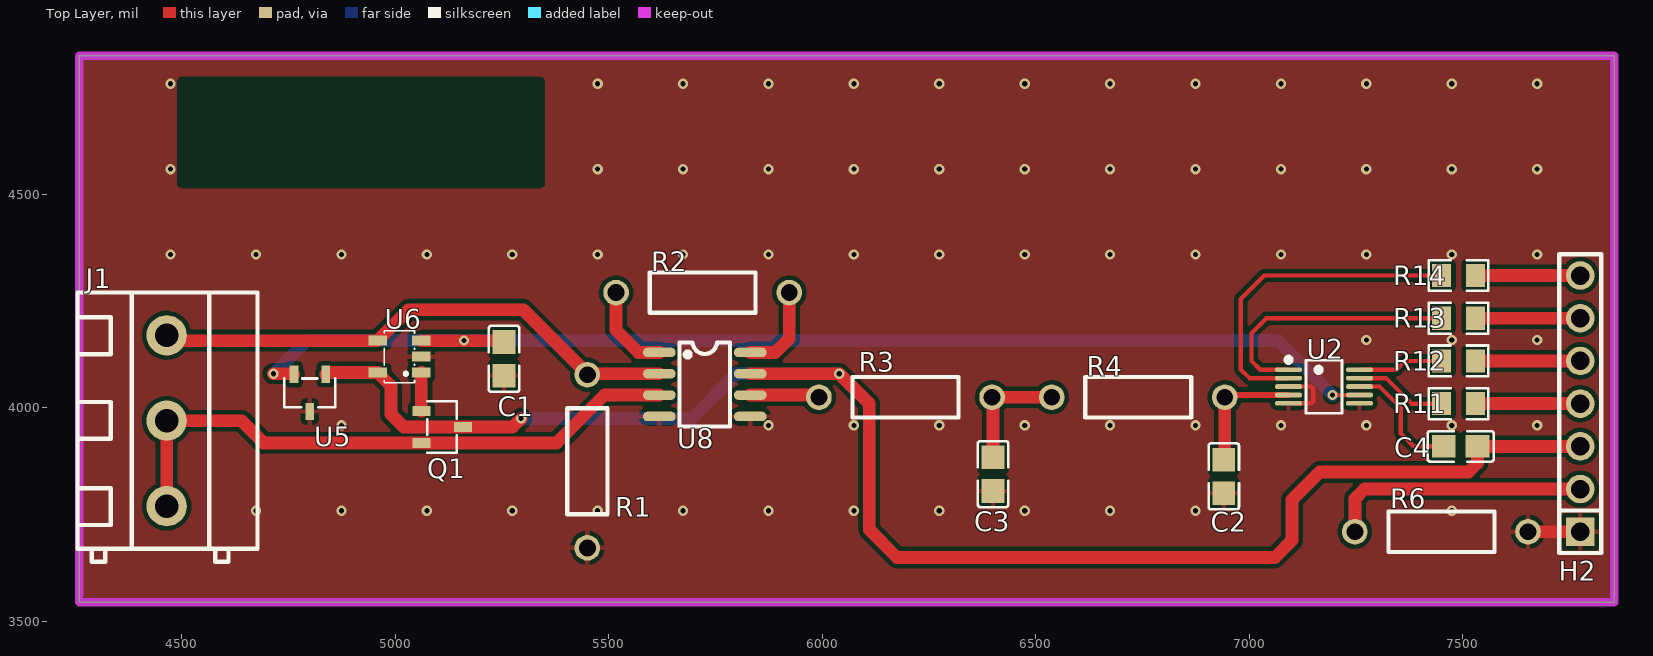
[diagram p0: Top Layer view]
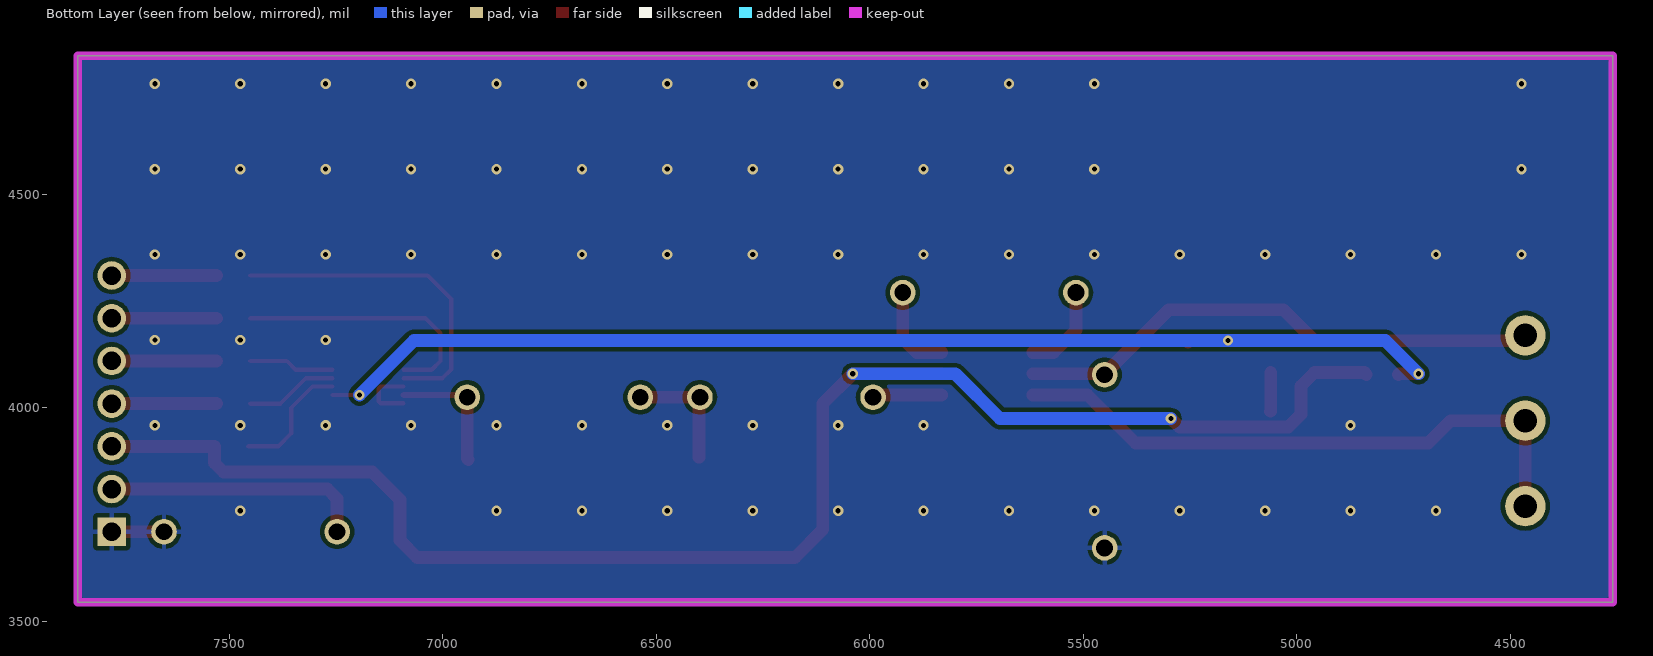
[diagram p1: Bottom Layer view, seen from below]
# Altium PCB MISC51892.pcbdoc
Units mil, origin at the board's own origin, x right, y up, seen from the top; angles counter-clockwise.
Board outline 3595 x 1280 mil, 2 copper layers (Top Layer, Bottom Layer), stack 62.206 mil thick; 20 components, 21 nets, 65 pads, 75 vias.

## Layer stack, top to bottom
Top Solder Mask Layer: solder mask 0.394, Dk 3.3
Top Layer: signal copper 1.379
Dielectric1: surface 59.449, FR4, Dk 4.5
Bottom Layer: signal copper 1.378
Bottom Solder Mask Layer: solder mask 0.394, Dk 3.3

## Board outline
4260,4825 4260,3545 7855,3545 7855,4825

## Design rules (kind name [scope] priority, off if disabled: settings)
BoardOutlineClearance copperThickness2oz_1 [All] p2 off: genericclearance=7.99 ignorepadtopadclearanceinfootprint=FALSE except(0: Arc-SplitContinuation Track-SplitContinuation SMDPad-SplitContinuation THPad-SplitContinuation Via-SplitContinuation Fill-SplitContinuation Region-SplitContinuation Poly-SplitContinuation Text-SplitContinuation Hole-SplitContinuation; 5.98: Arc-CutoutEdge Track-CutoutEdge SMDPad-CutoutEdge THPad-CutoutEdge Via-CutoutEdge Text-CutoutEdge; 6.9: Hole-OutlineEdge Hole-CutoutEdge; 10: Poly-OutlineEdge Poly-CutoutEdge; 11.81: Arc-OutlineEdge Track-OutlineEdge SMDPad-OutlineEdge THPad-OutlineEdge Via-OutlineEdge Fill-OutlineEdge Region-OutlineEdge Text-OutlineEdge Fill-CutoutEdge Region-CutoutEdge)
BoardOutlineClearance Plane_innerPlane_1 [All] p4 off: genericclearance=4.02 ignorepadtopadclearanceinfootprint=FALSE except(0: Arc-SplitContinuation Track-SplitContinuation SMDPad-SplitContinuation THPad-SplitContinuation Via-SplitContinuation Fill-SplitContinuation Region-SplitContinuation Poly-SplitContinuation Text-SplitContinuation Hole-SplitContinuation; 5.98: Arc-CutoutEdge Track-CutoutEdge SMDPad-CutoutEdge THPad-CutoutEdge Via-CutoutEdge Text-CutoutEdge; 6.9: Hole-OutlineEdge Hole-CutoutEdge; 10: Poly-OutlineEdge Poly-CutoutEdge; 11.81: Arc-OutlineEdge Track-OutlineEdge SMDPad-OutlineEdge THPad-OutlineEdge Via-OutlineEdge Fill-OutlineEdge Region-OutlineEdge Text-OutlineEdge Fill-CutoutEdge Region-CutoutEdge)
BoardOutlineClearance Copper_copperRegion_1 [All] p6 off: genericclearance=4.02 ignorepadtopadclearanceinfootprint=FALSE except(0: Arc-SplitContinuation Track-SplitContinuation SMDPad-SplitContinuation THPad-SplitContinuation Via-SplitContinuation Fill-SplitContinuation Region-SplitContinuation Poly-SplitContinuation Text-SplitContinuation Hole-SplitContinuation; 5.98: Arc-CutoutEdge Track-CutoutEdge SMDPad-CutoutEdge THPad-CutoutEdge Via-CutoutEdge Text-CutoutEdge; 6.9: Hole-OutlineEdge Hole-CutoutEdge; 10: Poly-OutlineEdge Poly-CutoutEdge; 11.81: Arc-OutlineEdge Track-OutlineEdge SMDPad-OutlineEdge THPad-OutlineEdge Via-OutlineEdge Fill-OutlineEdge Region-OutlineEdge Text-OutlineEdge Fill-CutoutEdge Region-CutoutEdge)
BoardOutlineClearance copperThickness1oz_1 [All] p8: genericclearance=4.02 ignorepadtopadclearanceinfootprint=FALSE except(0: Arc-SplitContinuation Track-SplitContinuation SMDPad-SplitContinuation THPad-SplitContinuation Via-SplitContinuation Fill-SplitContinuation Region-SplitContinuation Poly-SplitContinuation Text-SplitContinuation Hole-SplitContinuation; 5.98: Arc-CutoutEdge Track-CutoutEdge SMDPad-CutoutEdge THPad-CutoutEdge Via-CutoutEdge Text-CutoutEdge; 6.9: Hole-OutlineEdge Hole-CutoutEdge; 10: Poly-OutlineEdge Poly-CutoutEdge; 11.81: Arc-OutlineEdge Track-OutlineEdge SMDPad-OutlineEdge THPad-OutlineEdge Via-OutlineEdge Fill-OutlineEdge Region-OutlineEdge Text-OutlineEdge Fill-CutoutEdge Region-CutoutEdge)
Clearance copperThickness2oz [All] p1 off: gap=7.99 ignorepadtopadclearanceinfootprint=FALSE except(5.98: SMDPad-Track SMDPad-SMDPad THPad-Track SMDPad-THPad THPad-THPad Track-Via SMDPad-Via THPad-Via Via-Via Fill-SMDPad Region-SMDPad Fill-THPad Region-THPad Fill-Via Region-Via Fill-Fill Fill-Region Region-Region Arc-Track Arc-SMDPad Arc-THPad Arc-Via Fill-Arc Region-Arc Arc-Arc Text-Track SMDPad-Text Text-THPad Text-Via Fill-Text Region-Text Arc-Text Text-Text; 6.9: Hole-Track Hole-SMDPad Hole-THPad Hole-Via Fill-Hole Region-Hole Hole-Arc Hole-Text; 10: Poly-Track Poly-SMDPad Poly-THPad Poly-Via Poly-Fill Poly-Region Poly-Poly Poly-Arc Poly-Text Poly-Hole; 11.81: Fill-Track Region-Track)
Clearance Plane_innerPlane [All] p3 off: gap=4.02 ignorepadtopadclearanceinfootprint=FALSE except(5.98: SMDPad-Track SMDPad-SMDPad THPad-Track SMDPad-THPad THPad-THPad Track-Via SMDPad-Via THPad-Via Via-Via Fill-SMDPad Region-SMDPad Fill-THPad Region-THPad Fill-Via Region-Via Fill-Fill Fill-Region Region-Region Arc-Track Arc-SMDPad Arc-THPad Arc-Via Fill-Arc Region-Arc Arc-Arc Text-Track SMDPad-Text Text-THPad Text-Via Fill-Text Region-Text Arc-Text Text-Text; 6.9: Hole-Track Hole-SMDPad Hole-THPad Hole-Via Fill-Hole Region-Hole Hole-Arc Hole-Text; 10: Poly-Track Poly-SMDPad Poly-THPad Poly-Via Poly-Fill Poly-Region Poly-Poly Poly-Arc Poly-Text Poly-Hole; 11.81: Fill-Track Region-Track)
Clearance Copper_copperRegion [All] p5 off: gap=4.02 ignorepadtopadclearanceinfootprint=FALSE except(5.98: SMDPad-Track SMDPad-SMDPad THPad-Track SMDPad-THPad THPad-THPad Track-Via SMDPad-Via THPad-Via Via-Via Fill-SMDPad Region-SMDPad Fill-THPad Region-THPad Fill-Via Region-Via Fill-Fill Fill-Region Region-Region Arc-Track Arc-SMDPad Arc-THPad Arc-Via Fill-Arc Region-Arc Arc-Arc Text-Track SMDPad-Text Text-THPad Text-Via Fill-Text Region-Text Arc-Text Text-Text; 6.9: Hole-Track Hole-SMDPad Hole-THPad Hole-Via Fill-Hole Region-Hole Hole-Arc Hole-Text; 10: Poly-Track Poly-SMDPad Poly-THPad Poly-Via Poly-Fill Poly-Region Poly-Poly Poly-Arc Poly-Text Poly-Hole; 11.81: Fill-Track Region-Track)
Clearance copperThickness1oz [All] p7: gap=4.02 ignorepadtopadclearanceinfootprint=FALSE except(5.98: SMDPad-Track SMDPad-SMDPad THPad-Track SMDPad-THPad THPad-THPad Track-Via SMDPad-Via THPad-Via Via-Via Fill-SMDPad Region-SMDPad Fill-THPad Region-THPad Fill-Via Region-Via Fill-Fill Fill-Region Region-Region Arc-Track Arc-SMDPad Arc-THPad Arc-Via Fill-Arc Region-Arc Arc-Arc Text-Track SMDPad-Text Text-THPad Text-Via Fill-Text Region-Text Arc-Text Text-Text; 6.9: Hole-Track Hole-SMDPad Hole-THPad Hole-Via Fill-Hole Region-Hole Hole-Arc Hole-Text; 10: Poly-Track Poly-SMDPad Poly-THPad Poly-Via Poly-Fill Poly-Region Poly-Poly Poly-Arc Poly-Text Poly-Hole; 11.81: Fill-Track Region-Track)
DiffPairsRouting differentialPair [All] p1: maxlimit=6 minlimit=6 mostfreqgap=6 toplayer_minwidth=5 toplayer_prefwidth=10 toplayer_maxwidth=100 toplayer_mingap=6 toplayer_prefgap=6 toplayer_maxgap=6 bottomlayer_minwidth=5 bottomlayer_prefwidth=10 bottomlayer_maxwidth=100 bottomlayer_mingap=6 bottomlayer_prefgap=6 bottomlayer_maxgap=6 maxuncoupledlength=10
HoleToHoleClearance otherClearance [All] p1: gap=11.81 allowstackedmicrovias=TRUE
Length netLength [All] p1: minlimit=0 maxlimit=0
PasteMaskExpansion pasteMaskExpansion [All] p1: expansion=0
PlaneConnect innerPlane [All] p1: planeconnectstyle=Relief reliefexpansion=20 reliefentries=4 reliefconductorwidth=10 reliefairgap=10
PolygonConnect copperRegion [All] p1: connectstyle=Relief reliefconductorwidth=10 reliefentries=4 polygonreliefangle="90 Angle" airgapwidth=10 via.connectstyle=Relief via.reliefconductorwidth=10 via.reliefentries=4 via.polygonreliefangle="90 Angle" via.airgapwidth=10
RoutingVias viaSize [All] p1: holewidth=12.01 width=24.02 viastyle="Through Hole" minholewidth=11.81 minwidth=19.68 maxholewidth=248.03 maxwidth=393.7
SolderMaskExpansion solderMaskExpansion [IsVia] p1: expansion=-1000 istentingtop=TRUE
SolderMaskExpansion solderMaskExpansion [All] p2: expansion=2 istentingtop=FALSE
Width copperThickness2oz_2 [All] p1 off: maxlimit=100 minlimit=8 preferedwidth=10
Width copperThickness1oz_2 [All] p2: maxlimit=100 minlimit=5 preferedwidth=10

## Components (designator, comment, footprint, x,y, rotation, side; value= is the part's Value field where it differs from the comment)
C1 "100nF" C0805 5255,4115 r90 top
C2 "100nF" C0805 6940.31,3839.57 r90 top
C3 "100nF" C0805 6400,3845 r90 top
C4 "100nF" C0805 7495,3910 r0 top
H2 "PZ254V-11-07P" HDR-TH_7P-P2.54-V-M 7775,4010 r90 top
J1 "KF128-5.08-3P-AA" CONN-TH_3P-P5.08_KF128-5.08-3P 4465,3970 r270 top
Q1 "2N7002K-T1-GE3" SOT-23-3_L2.9-W1.6-P1.90-LS2.8-BR 5110,3955 r180 top
R1 "3.3kΩ" Res_1/4W 5450,3875 r90 top
R2 "3.3kΩ" Res_1/4W 5720,4270 r0 top
R3 "200" Res_1/4W 6195,4025 r0 top
R4 "200" Res_1/4W 6740,4025 r0 top
R6 "10K" Res_1/4W 7450,3710 r0 top
R11 "50" R0805 7490,4010 r0 top
R12 "50" R0805 7490,4110 r0 top
R13 "50" R0805 7490,4210 r0 top
R14 "50" R0805 7490,4310 r0 top
U2 "GD30AD3344" MSOP-10_L3.0-W3.0-P0.50-LS5.0-BL 7175,4050 r270 top
U5 "REF3033AIDBZR" SOT-23-3_L3.0-W1.7-P0.95-LS2.9-BR 4800,4035 r90 top
U6 "OPA333AIDBVR" SOT-23-5_L3.0-W1.7-P0.95-LS2.8-BR 5010,4120 r0 top
U8 "AD623ARZ-R7" SOIC-8_L5.0-W4.0-P1.27-LS6.0-BL 5725,4055 r270 top

## Footprints (in the part's own frame and the unit in brackets; to place one, negate y for a bottom-side part, rotate by r counter-clockwise, add the part's x,y. Pads: shape width x height; smd on the part's side, far side on the other; paste and mask are expansions set on the pad)
C0805 [mm]
  rect 1.41x1.35 smd paste-100 mask+0.051: 1(-1,0) 2(1,0)
  silkscreen extent -1.96,-0.9 1.96,0.9
CONN-TH_3P-P5.08_KF128-5.08-3P [mm]
  round 2.4 hole 1.4: 1(-5.08,0) 2(0,0) 3(5.08,0)
  silkscreen extent -7.62,-5.3 8.38,5.4
HDR-TH_7P-P2.54-V-M [mm]
  rect 1.7x1.7 hole 1.1: 1(-7.62,0)
  round 1.7 hole 1.1: 2(-5.08,0) 3(-2.54,0) 4(0,0) 5(2.54,0) 6(5.08,0) 7(7.62,0)
  silkscreen extent -8.89,-1.25 8.89,1.25
MSOP-10_L3.0-W3.0-P0.50-LS5.0-BL [mm]
  oval 0.28x1.62 smd: 1(-1,-2.11) 2(-0.5,-2.11) 3(0,-2.11) 4(0.5,-2.11) 5(1,-2.11) 6(1,2.11) 7(0.5,2.11) 8(0,2.11) 9(-0.5,2.11) 10(-1,2.11)
  silkscreen extent -1.74,-2.26 1.58,1.07
R0805 [mm]
  rect 1.133x1.377 smd paste-100 mask+0.051: 1(-1,0) 2(1,0)
  silkscreen extent -1.76,-0.92 1.76,0.92
Res_1/4W [mil]
  round 60 hole 39.37 paste+0 mask+2: 1(-202.76,0) 2(202.76,0)
  silkscreen extent -124,-47 124,47
SOIC-8_L5.0-W4.0-P1.27-LS6.0-BL [mil]
  oval 22.38x76.78 smd: 1(-75,-106.5) 2(-25,-106.5) 3(25,-106.5) 4(75,-106.5) 5(75,106.5) 6(25,106.5) 7(-25,106.5) 8(-75,106.5)
  silkscreen extent -98,-59 98,59
SOT-23-3_L2.9-W1.6-P1.90-LS2.8-BR [mm]
  rect 1.07x0.6 smd: 1(1.235,-0.95) 2(1.235,0.95) 3(-1.235,0)
  silkscreen extent -0.88,-1.54 0.88,1.54
SOT-23-3_L3.0-W1.7-P0.95-LS2.9-BR [mil]
  rect 40.85x20.95 smd: 1(43.36,-37.4) 2(43.36,37.4) 3(-43.36,0)
  silkscreen extent -34,-60 34,60
SOT-23-5_L3.0-W1.7-P0.95-LS2.8-BR [mm]
  rect 1.1x0.6 smd: 1(1.3,-0.95) 2(1.3,0) 3(1.3,0.95) 4(-1.3,0.95) 5(-1.3,-0.95)
  silkscreen extent -0.9,-1.55 0.9,1.55

## Via types
v1: diameter 24.02, hole 12, Top Layer to Bottom Layer, 75 vias

## Nets (pads, with @x,y where several pads share a name; then routed paths per layer and width w, separated by ;. In a path a pad name is that pad's centre, name@x,y a point inside that pad or via, vN(x,y) a via of type N, cw(c..) or ccw(c..) an arc to the next point about the centre after c; other vN are vias at no path point)
3.3V: C1.2 U2.7 U5.2 U6.3 | length 2871.6
  Top Layer w10: v1(7195,4030.31) U2.7
  Top Layer w30: v1(4715,4080) 4760.96,4080 U5.2 ; U6.3 5251.97,4157.4 C1.2
  Bottom Layer w30: v1(4715,4080) 4793,4158 v1(5161,4158) 7067.31,4158 v1(7195,4030.31)
$1N932: J1.2 J1.3 Q1.2 U8.3 | length 1421.8
  Top Layer w30: J1.3 J1.2 4640,3970 4692.4,3917.6 Q1.2 5377.6,3917.6 5490,4030 U8.3
$1N951: J1.1 R1.2 U6.4 U8.2 | length 1254.1
  Top Layer w30: J1.1 4477.6,4157.4 U6.4 5031.41,4230 5300,4230 5450,4080 R1.2 5452.24,4080 U8.2
$1N1020: Q1.1 U6.1 | length 90.3
  Top Layer w30: U6.1 5061.19,3992.59 Q1.1
$1N1082: R2.1 U8.1 | length 210.4
  Top Layer w30: R2.1 5517.24,4182.76 5570,4130 U8.1
$1N1087: R2.2 U8.8 | length 212.1
  Top Layer w30: U8.8 5890,4130 5922.76,4162.76 R2.2
$1N1302: R3.1 U8.6 | length 162.8
  Top Layer w30: U8.6 5987.24,4030 R3.1
$1N1306: C3.2 R3.2 R4.1 | length 281
  Top Layer w30: C3.2 6400,4022.76 R3.2 R4.1
$1N1602: C2.2 R4.2 U2.4 | length 298.4
  Top Layer w15: R4.2 6948.07,4030.31 U2.4
  Top Layer w30: C2.2 6942.76,3881.4 R4.2
$1N3512: C4.1 U2.8 | length 290.7
  Top Layer w10: U2.8 7305,4050 7355,4000 7355,3940 7385,3910 C4.1
$1N3802: H2.4 R11.2 | length 245.6
  Top Layer w30: R11.2 H2.4
$1N3804: H2.5 R12.2 | length 245.6
  Top Layer w30: R12.2 H2.5
$1N3806: H2.6 R13.2 | length 245.6
  Top Layer w30: R13.2 H2.6
$1N3808: H2.7 R14.2 | length 245.6
  Top Layer w30: R14.2 H2.7
+5V: C4.2 H2.3 Q1.3 U5.1 U6.5 U8.7 | length 3828.3
  Top Layer w30: U5.1 4841.64,4082.6 U6.5 4990,4051.41 4990,3985 5020,3955 Q1.3 5275,3955 v1(5295,3975) ; U8.7 v1(6040,4080) 6110,4010 6110,3715 6175,3650 7060,3650 7100,3690 7100,3785 7165,3850 7513.1,3850 7534.37,3871.27 C4.2 H2.3
  Bottom Layer w30: v1(5295,3975) 5695,3975 5800,4080 v1(6040,4080)
AGND: C1.1 C2.1 C3.1 H2.1 R1.1 R6.2 U2.3 U2.5 U2.6 U5.3 U6.2 U8.4 U8.5 | length 272.3
  Top Layer w10: U2.5 7145.63,4010.63 7150,4015 7150,4045 7145,4050 U2.3
  Top Layer w30: R6.2 H2.1
  other v1: 4674.1,3759.1 4874.1,3759.1 5074.1,3759.1 5274.1,3759.1 5474.1,3759.1 5674.1,3759.1 5874.1,3759.1 6074.1,3759.1 6274.1,3759.1 6474.1,3759.1 6674.1,3759.1 6874.1,3759.1 7474.1,3759.1 4874.1,3959.1 5874.1,3959.1 6074.1,3959.1 6274.1,3959.1 6474.1,3959.1 6674.1,3959.1 6874.1,3959.1 7074.1,3959.1 7274.1,3959.1 7474.1,3959.1 7674.1,3959.1 7274.1,4159.1 7474.1,4159.1 7674.1,4159.1 4474.1,4359.1 4674.1,4359.1 4874.1,4359.1 5074.1,4359.1 5274.1,4359.1 5474.1,4359.1 5674.1,4359.1 5874.1,4359.1 6074.1,4359.1 6274.1,4359.1 6474.1,4359.1 6674.1,4359.1 6874.1,4359.1 7074.1,4359.1 7274.1,4359.1 7474.1,4359.1 7674.1,4359.1 4474.1,4559.1 5474.1,4559.1 5674.1,4559.1 5874.1,4559.1 6074.1,4559.1 6274.1,4559.1 6474.1,4559.1 6674.1,4559.1 6874.1,4559.1 7074.1,4559.1 7274.1,4559.1 7474.1,4559.1 7674.1,4559.1 4474.1,4759.1 5474.1,4759.1 5674.1,4759.1 5874.1,4759.1 6074.1,4759.1 6274.1,4759.1 6474.1,4759.1 6674.1,4759.1 6874.1,4759.1 7074.1,4759.1 7274.1,4759.1 7474.1,4759.1 7674.1,4759.1
GND: H2.2 R6.1 | length 614.4
  Top Layer w30: R6.1 7247.24,3787.24 7270,3810 H2.2
SPICLK: R13.1 U2.1 | length 620.6
  Top Layer w10: U2.1 7025.63,4089.37 7005,4110 7005,4175 7040,4210 R13.1
SPIMISO: R11.1 U2.9 | length 217.3
  Top Layer w10: U2.9 7320.32,4069.68 7380,4010 R11.1
SPIMOSI: R12.1 U2.10 | length 201.1
  Top Layer w10: U2.10 7344.37,4089.37 7365,4110 R12.1
SPINSS: R14.1 U2.2 | length 778.8
  Top Layer w10: U2.2 7000.32,4069.68 6980,4090 6980,4255 7035,4310 R14.1

## Polygon pours and split planes (outlines as drawn)
AGND on Top Layer (solid, remove dead copper, pour order 0): 3000,5285 3000,3000 7940,3000 7940,5285
AGND on Bottom Layer (solid, remove dead copper, pour order 2): 3000,5325 3000,3035 7885,3035 7885,5325

## Keep-outs
Board Outline Layer:
  the board outline again, w20